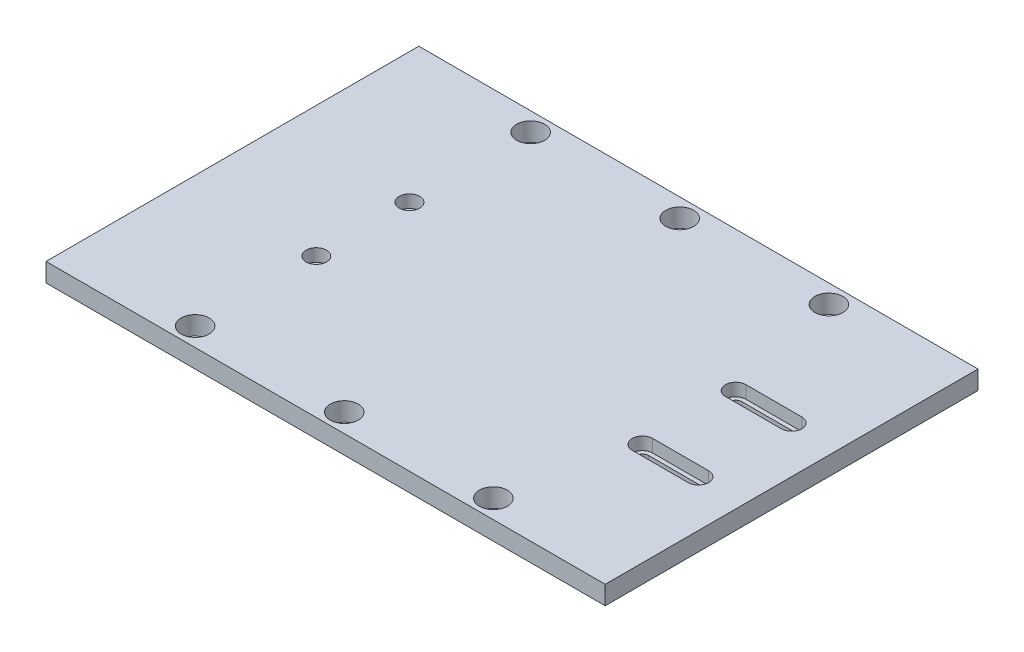
SolidWorks part; units mm, degrees
ref_plane "Front Plane" through (0, 0, 0) normal (0, 0, 1) x (1, 0, 0)
ref_plane "Top Plane" through (0, 0, 0) normal (0, 1, 0) x (1, 0, 0)
ref_plane "Right Plane" through (0, 0, 0) normal (1, 0, 0) x (0, 0, -1)
sketch "Sketch1" plane through (0, 0, 0) normal (0, 1, 0) x (1, 0, 0)
  line L1 (-150, 100) -> (150, 100)
  line L2 (-150, 100) -> (-150, -100)
  line L3 (-150, -100) -> (150, -100)
  line L4 (150, 100) -> (150, -100)
  line L5 (-150, 100) -> (150, -100) construction
  line L6 (-150, -100) -> (150, 100) construction
  point P0 (0, 0)
  dimension "D1" = 200
  dimension "D2" = 300
extrude "Boss-Extrude1" add sketch "Sketch1" along normal mid plane 10
sketch "Sketch2" plane through (0, 5, 0) normal (0, 1, 0) x (1, 0, 0)
  line L0 (0, 90) -> (0, -90) construction
  line L1 (80, 90) -> (-80, 90) construction
  line L2 (80, 90) -> (80, -90) construction
  line L3 (80, -90) -> (-80, -90) construction
  line L4 (-80, 90) -> (-80, -90) construction
  line L5 (80, 90) -> (-80, -90) construction
  line L6 (80, -90) -> (-80, 90) construction
  circle A0 centre (80, 90) radius 7.5
  point P0 (0, 0)
  dimension "D3" = 15
  dimension "D1" = 180
  dimension "D2" = 160
extrude "Cut-Extrude1" cut sketch "Sketch2" against normal blind 10
pattern_linear "LPattern1" count 2 spacing 180 along (0, 0, 1) count 3 spacing 80 along (-1, 0, 0) of "Cut-Extrude1"
sketch "Sketch3" plane through (0, 5, 0) normal (0, 1, 0) x (1, 0, 0)
  line L0 (15, 0) -> (0, 0) construction
  line L1 (110, 25) -> (-80, 25) construction
  line L2 (110, 25) -> (110, -25) construction
  line L3 (110, -25) -> (-80, -25) construction
  line L4 (-80, 25) -> (-80, -25) construction
  line L5 (110, 25) -> (-80, -25) construction
  line L6 (110, -25) -> (-80, 25) construction
  point P0 (15, 0)
  dimension "D1" = 50
  dimension "D2" = 190
  dimension "D3" = 80
hole_wizard "Hole Size (based on socket head cap screw type)1" positions "Sketch4" profile "Sketch5" counterbore size "M6" standard "GB" end condition up to next
sketch "Sketch4" plane through (0, 5, 0) normal (0, 1, 0) x (1, 0, 0)
  point P6 (-80, 25)
  point P9 (-80, -25)
sketch "Sketch5" plane through (-80, 5, -25) normal (1, 0, 0) x (0, 0, 1)
  line L0 (0, 0) -> (0, 10)
  line L1 (0, 10) -> (3.3, 10)
  line L3 (3.3, 10) -> (3.3, 6.8)
  line L4 (3.3, 6.8) -> (5.5, 6.8)
  line L5 (5.5, 6.8) -> (5.5, 0)
  line L7 (5.5, 0) -> (0, 0)
  line L11 (0, -6.35) -> (0, 107.95) construction
  dimension "通孔孔直径" = 6.6
  dimension "通孔孔深度" = 10
  dimension "柱形沉头孔直径" = 11
  dimension "柱形沉头孔深度" = 6.8
sketch "Sketch6" plane through (0, 5, 0) normal (0, 1, 0) x (1, 0, 0)
  line L0 (125, 25) -> (95, 25) construction
  line L1 (110, 25) -> (-80, 25) construction
  line L2 (125, 21.7) -> (95, 21.7)
  line L3 (125, 28.3) -> (95, 28.3)
  line L4 (125, -25) -> (95, -25) construction
  line L5 (110, -25) -> (-80, -25) construction
  line L6 (125, -28.3) -> (95, -28.3)
  line L7 (125, -21.7) -> (95, -21.7)
  arc A0 (125, 21.7) -> (125, 28.3) centre (125, 25) ccw
  arc A1 (95, 28.3) -> (95, 21.7) centre (95, 25) ccw
  arc A2 (125, -28.3) -> (125, -21.7) centre (125, -25) ccw
  arc A3 (95, -21.7) -> (95, -28.3) centre (95, -25) ccw
  point P5 (110, 25)
  point P15 (110, -25)
  dimension "D1" = 3.3
  dimension "D2" = 3.3
  dimension "D3" = 30
  dimension "D4" = 30
extrude "Cut-Extrude2" cut sketch "Sketch6" against normal blind 10
sketch "Sketch7" plane through (0, 5, 0) normal (0, 1, 0) x (1, 0, 0)
  line L0 (125, 25) -> (95, 25) construction
  line L1 (110, 25) -> (-80, 25) construction
  line L2 (125, 19.5) -> (95, 19.5)
  line L3 (125, 30.5) -> (95, 30.5)
  line L4 (125, -25) -> (95, -25) construction
  line L5 (110, -25) -> (-80, -25) construction
  line L6 (125, -30.5) -> (95, -30.5)
  line L7 (125, -19.5) -> (95, -19.5)
  arc A0 (125, 19.5) -> (125, 30.5) centre (125, 25) ccw
  arc A1 (95, 30.5) -> (95, 19.5) centre (95, 25) ccw
  arc A2 (125, -30.5) -> (125, -19.5) centre (125, -25) ccw
  arc A3 (95, -19.5) -> (95, -30.5) centre (95, -25) ccw
  point P5 (110, 25)
  point P11 (110, -25)
  dimension "D3" = 5.5
  dimension "D4" = 5.5
  dimension "D1" = 30
  dimension "D2" = 30
extrude "Cut-Extrude3" cut sketch "Sketch7" against normal blind 6.8
